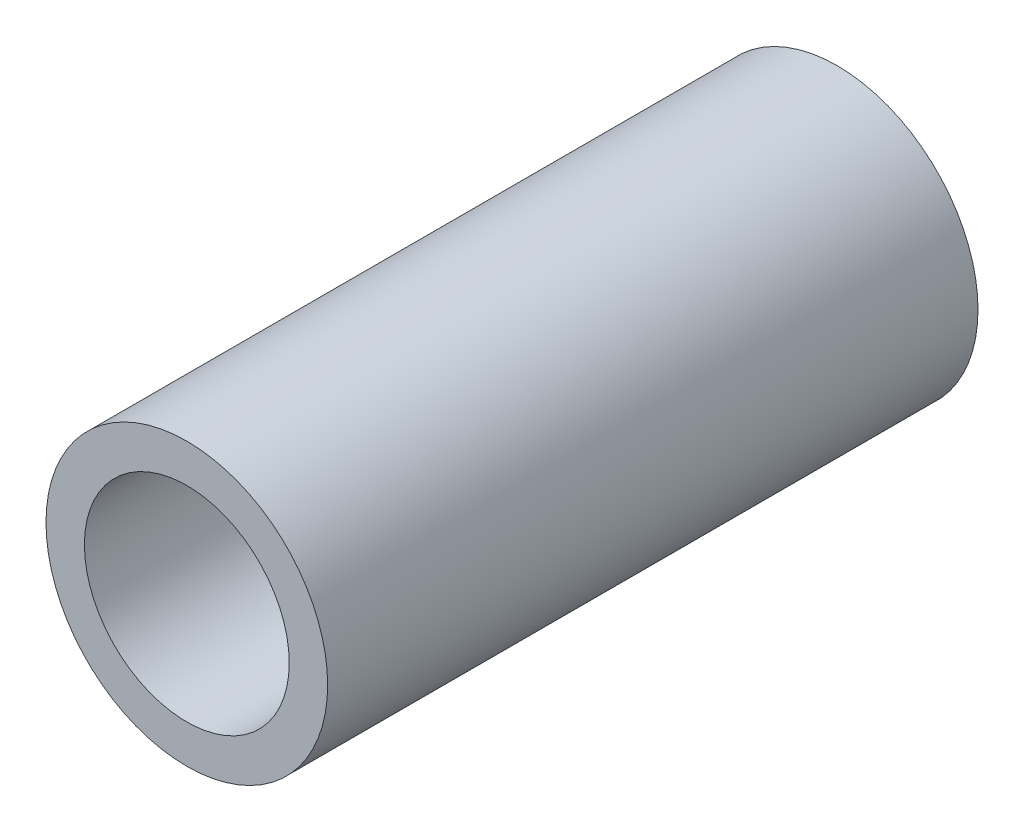
SolidWorks part; units mm, degrees
material "AISI 1020"
ref_plane "Front Plane" through (0, 0, 0) normal (0, 0, 1) x (1, 0, 0)
ref_plane "Top Plane" through (0, 0, 0) normal (0, 1, 0) x (1, 0, 0)
ref_plane "Right Plane" through (0, 0, 0) normal (1, 0, 0) x (0, 0, -1)
sketch "Sketch1" plane through (0, 0, 0) normal (0, 0, 1) x (1, 0, 0)
  circle A0 centre (0, 0) radius 11
  circle A1 centre (0, 0) radius 8
  dimension "D1" = 22
  dimension "D2" = 16
extrude "Extrude1" add sketch "Sketch1" along normal blind 50.8
